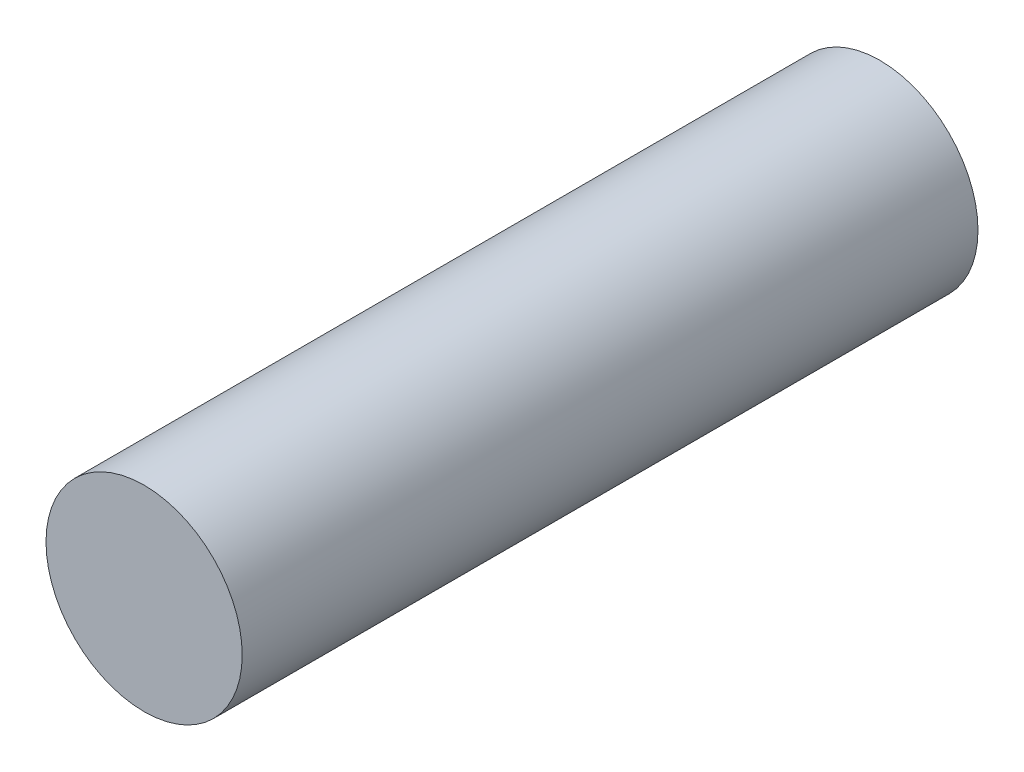
SolidWorks part; units mm, degrees
ref_plane "Front Plane" through (0, 0, 0) normal (0, 0, 1) x (1, 0, 0)
ref_plane "Top Plane" through (0, 0, 0) normal (0, 1, 0) x (1, 0, 0)
ref_plane "Right Plane" through (0, 0, 0) normal (1, 0, 0) x (0, 0, -1)
other "Configuration Table"
sketch "Sketch1" plane through (0, 0, 0) normal (0, 0, 1) x (1, 0, 0)
  circle A0 centre (0, 0) radius 12
  dimension "D1" = 24
extrude "Boss-Extrude1" add sketch "Sketch1" along normal blind 90
